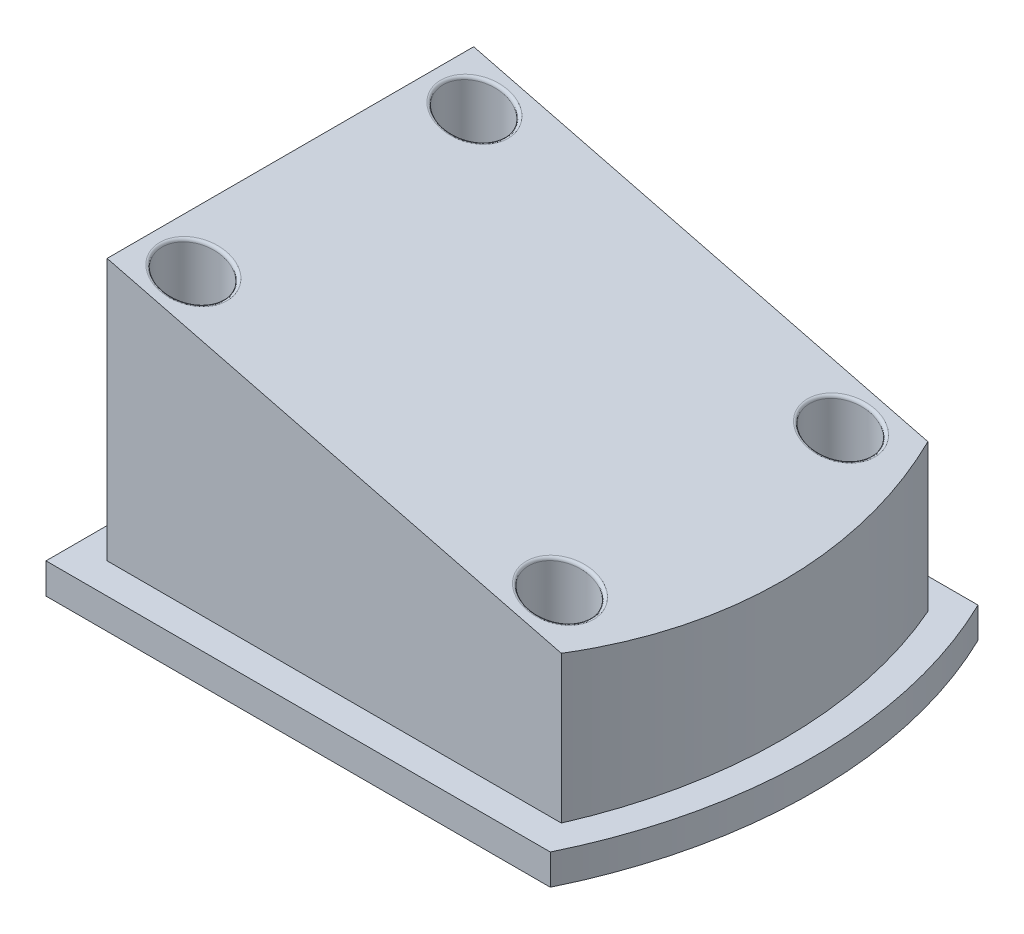
from build123d import *

# Parameters (mm, degrees)
BOSS_EXTRUDE1_DEPTH     = 5
BOSS_EXTRUDE2_DEPTH     = 42.87
CUT_EXTRUDE1_DEPTH      = 95.605682361
CUT_EXTRUDE1_DEPTH_BACK = 95.605682361
CUT_EXTRUDE2_REACH      = 99.138
CUT_EXTRUDE2_START      = -20
SKETCH5_R               = 5
CUT_EXTRUDE3_REACH      = 81.139
CUT_EXTRUDE3_START      = 5
SKETCH6_R               = 3
FILLET1_R               = 0.5


with BuildPart() as part:
    # Sketch1 → Boss-Extrude1 (new body)
    with BuildSketch(Plane(origin=(0, 0, 0), x_dir=(1, 0, 0), z_dir=(0, 1, 0))):
        with BuildLine():
            Line((-41.27, 35), (41.27, 35))
            ThreePointArc((41.27, 35), (49.33252715, 0), (41.27, -35))
            Line((41.27, -35), (-41.27, -35))
            Line((-41.27, -35), (-41.27, 35))
        make_face()
    extrude(amount=BOSS_EXTRUDE1_DEPTH)

    # Sketch2 → Boss-Extrude2 (add)
    with BuildSketch(Plane(origin=(0, 5, 0), x_dir=(1, 0, 0), z_dir=(0, 1, 0))):
        with BuildLine():
            Line((38.071162575, 30), (-36.27, 30))
            Line((-36.27, 30), (-36.27, -30))
            Line((-36.27, -30), (38.071162575, -30))
            ThreePointArc((38.071162575, -30), (44.33252715, 0), (38.071162575, 30))
        make_face()
    extrude(amount=BOSS_EXTRUDE2_DEPTH)

    # Sketch3 → Cut-Extrude1 (cut, two sides: drawn at the far end of the back side and taken through both)
    with BuildSketch(Plane.XY.offset(30).offset(-CUT_EXTRUDE1_DEPTH_BACK)):
        Polygon((44.33252715, -196.474588962), (44.33252715, 5), (44.33252715, 27.48), (-36.27, 47.87), (-36.27, 5), (-36.27, -196.474588962), (-36.27, 206.474588962), (44.33252715, 206.474588962), align=None)
    extrude(amount=CUT_EXTRUDE1_DEPTH + CUT_EXTRUDE1_DEPTH_BACK, mode=Mode.SUBTRACT)

    # Cut-Extrude2: up to this plane
    cut_extrude2_end = Plane(origin=(-36.27, 47.87, 266.372707608), z_dir=(-0.24524436739565725, -0.9694612938434953, 0))
    # Sketch5 → Cut-Extrude2 (cut, up to the surface)
    with BuildSketch(Plane.XZ.offset(CUT_EXTRUDE2_START), mode=Mode.PRIVATE) as cut_extrude2_sk1:
        with Locations(Location((-29.27, 23, 0), (0, 0, 270))):
            Circle(SKETCH5_R)
    cut_extrude2_tool1 = split(extrude(cut_extrude2_sk1.sketch, amount=-CUT_EXTRUDE2_REACH, mode=Mode.PRIVATE), bisect_by=cut_extrude2_end, keep=Keep.BOTH, mode=Mode.PRIVATE)
    add(cut_extrude2_tool1.solids().sort_by_distance((-29.27, 20, 23))[0], mode=Mode.SUBTRACT)
    # Sketch5 → Cut-Extrude2 (cut, up to the surface)
    with BuildSketch(Plane.XZ.offset(CUT_EXTRUDE2_START), mode=Mode.PRIVATE) as cut_extrude2_sk2:
        with Locations(Location((30.73, 23, 0), (0, 0, 270))):
            Circle(SKETCH5_R)
    cut_extrude2_tool2 = split(extrude(cut_extrude2_sk2.sketch, amount=-CUT_EXTRUDE2_REACH, mode=Mode.PRIVATE), bisect_by=cut_extrude2_end, keep=Keep.BOTH, mode=Mode.PRIVATE)
    add(cut_extrude2_tool2.solids().sort_by_distance((30.73, 20, 23))[0], mode=Mode.SUBTRACT)
    # Sketch5 → Cut-Extrude2 (cut, up to the surface)
    with BuildSketch(Plane.XZ.offset(CUT_EXTRUDE2_START), mode=Mode.PRIVATE) as cut_extrude2_sk3:
        with Locations((30.73, -23)):
            Circle(SKETCH5_R)
    cut_extrude2_tool3 = split(extrude(cut_extrude2_sk3.sketch, amount=-CUT_EXTRUDE2_REACH, mode=Mode.PRIVATE), bisect_by=cut_extrude2_end, keep=Keep.BOTH, mode=Mode.PRIVATE)
    add(cut_extrude2_tool3.solids().sort_by_distance((30.73, 20, -23))[0], mode=Mode.SUBTRACT)
    # Sketch5 → Cut-Extrude2 (cut, up to the surface)
    with BuildSketch(Plane.XZ.offset(CUT_EXTRUDE2_START), mode=Mode.PRIVATE) as cut_extrude2_sk4:
        with Locations((-29.27, -23)):
            Circle(SKETCH5_R)
    cut_extrude2_tool4 = split(extrude(cut_extrude2_sk4.sketch, amount=-CUT_EXTRUDE2_REACH, mode=Mode.PRIVATE), bisect_by=cut_extrude2_end, keep=Keep.BOTH, mode=Mode.PRIVATE)
    add(cut_extrude2_tool4.solids().sort_by_distance((-29.27, 20, -23))[0], mode=Mode.SUBTRACT)

    # Sketch6 → Cut-Extrude3 (cut, up to next)
    with BuildSketch(Plane(origin=(0, 5, 0), x_dir=(1, 0, 0), z_dir=(0, 1, 0)).offset(CUT_EXTRUDE3_START), mode=Mode.PRIVATE) as cut_extrude3_sk1:
        with Locations(Location((-29.27, 23, 0), (0, 0, 270))):
            Circle(SKETCH6_R)
    cut_extrude3_tool1 = extrude(cut_extrude3_sk1.sketch, amount=CUT_EXTRUDE3_REACH, mode=Mode.PRIVATE) & part.part
    # Sketch6 → Cut-Extrude3 (cut, up to next)
    with BuildSketch(Plane(origin=(0, 5, 0), x_dir=(1, 0, 0), z_dir=(0, 1, 0)).offset(CUT_EXTRUDE3_START), mode=Mode.PRIVATE) as cut_extrude3_sk2:
        with Locations(Location((30.73, 23, 0), (0, 0, 270))):
            Circle(SKETCH6_R)
    cut_extrude3_tool2 = extrude(cut_extrude3_sk2.sketch, amount=CUT_EXTRUDE3_REACH, mode=Mode.PRIVATE) & part.part
    # Sketch6 → Cut-Extrude3 (cut, up to next)
    with BuildSketch(Plane(origin=(0, 5, 0), x_dir=(1, 0, 0), z_dir=(0, 1, 0)).offset(CUT_EXTRUDE3_START), mode=Mode.PRIVATE) as cut_extrude3_sk3:
        with Locations(Location((-29.27, -23, 0), (0, 0, 90))):
            Circle(SKETCH6_R)
    cut_extrude3_tool3 = extrude(cut_extrude3_sk3.sketch, amount=CUT_EXTRUDE3_REACH, mode=Mode.PRIVATE) & part.part
    # Sketch6 → Cut-Extrude3 (cut, up to next)
    with BuildSketch(Plane(origin=(0, 5, 0), x_dir=(1, 0, 0), z_dir=(0, 1, 0)).offset(CUT_EXTRUDE3_START), mode=Mode.PRIVATE) as cut_extrude3_sk4:
        with Locations(Location((30.73, -23, 0), (0, 0, 90))):
            Circle(SKETCH6_R)
    cut_extrude3_tool4 = extrude(cut_extrude3_sk4.sketch, amount=CUT_EXTRUDE3_REACH, mode=Mode.PRIVATE) & part.part
    add(cut_extrude3_tool1.solids().sort_by_distance((-29.27, 10, -23))[0], mode=Mode.SUBTRACT)
    add(cut_extrude3_tool2.solids().sort_by_distance((30.73, 10, -23))[0], mode=Mode.SUBTRACT)
    add(cut_extrude3_tool3.solids().sort_by_distance((-29.27, 10, 23))[0], mode=Mode.SUBTRACT)
    add(cut_extrude3_tool4.solids().sort_by_distance((30.73, 10, 23))[0], mode=Mode.SUBTRACT)

    # Fillet1
    fillet1_edges = [part.edges().sort_by_distance(p)[0] for p in [
        (30.730000686, 30.921027526, 28),
        (25.73, 32.185876379, -23.000002484),
        (-34.27, 47.364060528, -23.000002484),
        (-29.269999314, 46.099211676, 28),
    ]]
    fillet(fillet1_edges, radius=FILLET1_R)


solid = part.part
